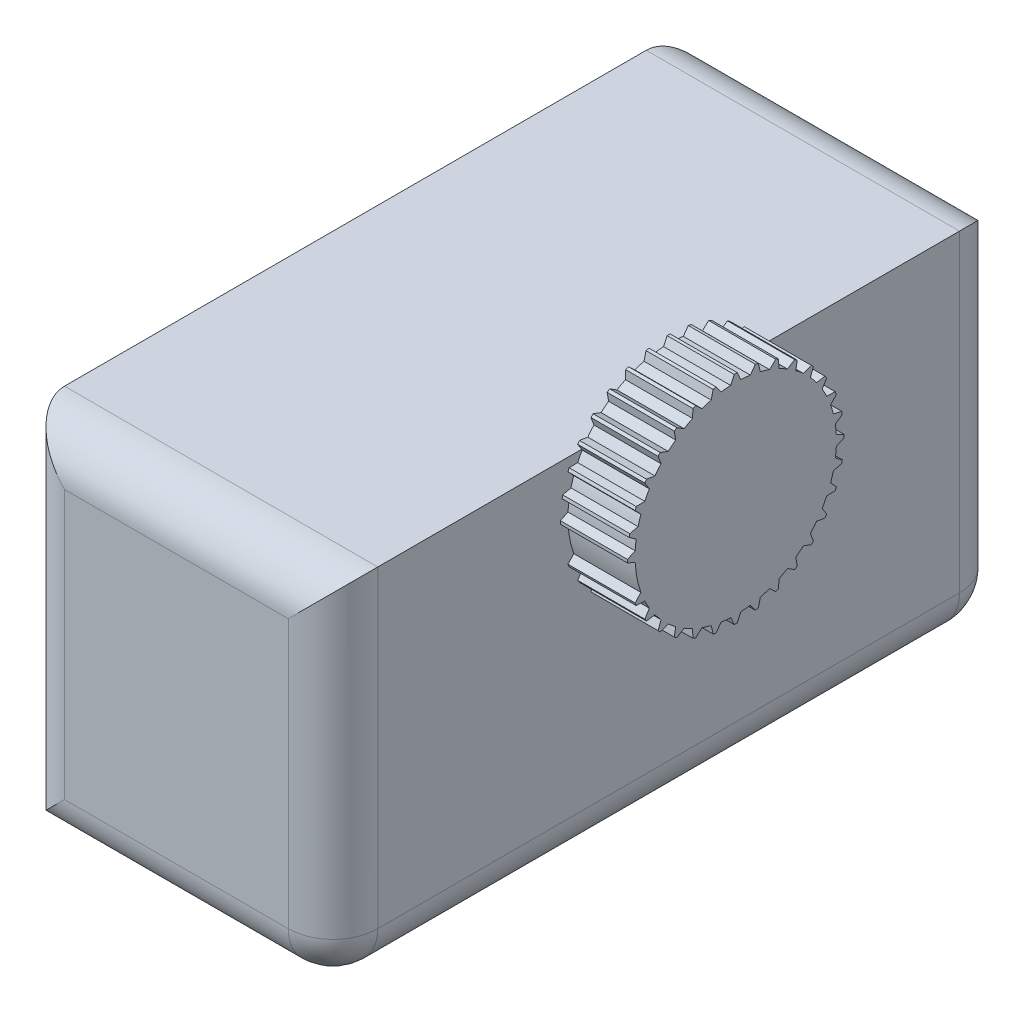
from build123d import *

# Parameters (mm, degrees)
SKETCH1_W                   = 28
SKETCH1_H                   = 32
BOSS_EXTRUDE1_DEPTH         = 30
BOSS_EXTRUDE3_DEPTH         = 6
FILLET1_R                   = 4
TAP_DRILL_FOR_M8_TAP1_D     = 6.8
TAP_DRILL_FOR_M8_TAP1_DEPTH = 5
TAP_DRILL_FOR_M8_TAP1_TIP   = 2.042926105


with BuildPart() as part:
    # Sketch1 → Boss-Extrude1 (new, symmetric)
    with BuildSketch(Plane.XY):
        Rectangle(SKETCH1_W, SKETCH1_H)
    extrude(amount=BOSS_EXTRUDE1_DEPTH, both=True)

    # Sketch2 → Boss-Extrude3 (add)
    with BuildSketch(Plane(origin=(14, 0, 0), x_dir=(0, 0, -1), z_dir=(1, 0, 0))):
        with BuildLine():
            Line((-0.137115518, 20.975970302), (0.137115518, 20.975970302))
            Line((0.137115518, 20.975970302), (0.450893035, 20.282586335))
            ThreePointArc((0.450893035, 20.282586335), (0.882154263, 20.250550667), (1.311378777, 20.197835887))
            Line((1.311378777, 20.197835887), (1.754399647, 20.816681719))
            Line((1.754399647, 20.816681719), (2.023361412, 20.763181898))
            Line((2.023361412, 20.763181898), (2.195837279, 20.021906152))
            ThreePointArc((2.195837279, 20.021906152), (2.612562095, 19.906351149), (3.023255037, 19.77091172))
            Line((3.023255037, 19.77091172), (3.578494218, 20.291437518))
            Line((3.578494218, 20.291437518), (3.83185066, 20.186493844))
            Line((3.83185066, 20.186493844), (3.856396729, 19.425813131))
            ThreePointArc((3.856396729, 19.425813131), (4.242570631, 19.231179507), (4.618949301, 19.01822029))
            Line((4.618949301, 19.01822029), (5.265069263, 19.42042254))
            Line((5.265069263, 19.42042254), (5.493084037, 19.268067939))
            Line((5.493084037, 19.268067939), (5.368757014, 18.517214793))
            ThreePointArc((5.368757014, 18.517214793), (5.709539557, 18.250982208), (6.037139934, 17.968687106))
            Line((6.037139934, 17.968687106), (6.749310649, 18.237109402))
            Line((6.749310649, 18.237109402), (6.943221275, 18.043198777))
            Line((6.943221275, 18.043198777), (6.674798979, 17.331028062))
            ThreePointArc((6.674798979, 17.331028062), (6.95709408, 17.003427685), (7.223326666, 16.662645142))
            Line((7.223326666, 16.662645142), (7.974179812, 16.786972164))
            Line((7.974179812, 16.786972164), (8.126534413, 16.558957391))
            Line((8.126534413, 16.558957391), (7.724332162, 15.912837429))
            ThreePointArc((7.724332162, 15.912837429), (7.937291379, 15.536458759), (8.131925004, 15.150284856))
            Line((8.131925004, 15.150284856), (8.892605716, 15.125738788))
            Line((8.892605716, 15.125738788), (8.997549391, 14.872382346))
            Line((8.997549391, 14.872382346), (8.477023592, 14.317143164))
            ThreePointArc((8.477023592, 14.317143164), (8.612463022, 13.906450223), (8.728018025, 13.489725407))
            Line((8.728018025, 13.489725407), (9.46929377, 13.317249539))
            Line((9.46929377, 13.317249539), (9.522793592, 13.048287775))
            Line((9.522793592, 13.048287775), (8.90394776, 12.605266904))
            ThreePointArc((8.90394776, 12.605266904), (8.95666254, 12.17604239), (8.988698208, 11.744781162))
            Line((8.988698208, 11.744781162), (9.682082175, 11.431003646))
            Line((9.682082175, 11.431003646), (9.682082175, 11.156772609))
            Line((9.682082175, 11.156772609), (8.988698208, 10.842995093))
            ThreePointArc((8.988698208, 10.842995093), (8.95666254, 10.411733864), (8.90394776, 9.982509351))
            Line((8.90394776, 9.982509351), (9.522793592, 9.53948848))
            Line((9.522793592, 9.53948848), (9.46929377, 9.270526716))
            Line((9.46929377, 9.270526716), (8.728018025, 9.098050848))
            ThreePointArc((8.728018025, 9.098050848), (8.612463022, 8.681326032), (8.477023592, 8.270633091))
            Line((8.477023592, 8.270633091), (8.997549391, 7.715393909))
            Line((8.997549391, 7.715393909), (8.892605716, 7.462037467))
            Line((8.892605716, 7.462037467), (8.131925004, 7.437491399))
            ThreePointArc((8.131925004, 7.437491399), (7.937291379, 7.051317496), (7.724332162, 6.674938826))
            Line((7.724332162, 6.674938826), (8.126534413, 6.028818864))
            Line((8.126534413, 6.028818864), (7.974179812, 5.80080409))
            Line((7.974179812, 5.80080409), (7.223326666, 5.925131113))
            ThreePointArc((7.223326666, 5.925131113), (6.95709408, 5.58434857), (6.674798979, 5.256748193))
            Line((6.674798979, 5.256748193), (6.943221275, 4.544577478))
            Line((6.943221275, 4.544577478), (6.749310649, 4.350666852))
            Line((6.749310649, 4.350666852), (6.037139934, 4.619089148))
            ThreePointArc((6.037139934, 4.619089148), (5.709539557, 4.336794047), (5.368757014, 4.070561462))
            Line((5.368757014, 4.070561462), (5.493084037, 3.319708316))
            Line((5.493084037, 3.319708316), (5.265069263, 3.167353714))
            Line((5.265069263, 3.167353714), (4.618949301, 3.569555965))
            ThreePointArc((4.618949301, 3.569555965), (4.242570631, 3.356596748), (3.856396729, 3.161963123))
            Line((3.856396729, 3.161963123), (3.83185066, 2.401282411))
            Line((3.83185066, 2.401282411), (3.578494218, 2.296338737))
            Line((3.578494218, 2.296338737), (3.023255037, 2.816864535))
            ThreePointArc((3.023255037, 2.816864535), (2.612562095, 2.681425106), (2.195837279, 2.565870102))
            Line((2.195837279, 2.565870102), (2.023361412, 1.824594357))
            Line((2.023361412, 1.824594357), (1.754399647, 1.771094536))
            Line((1.754399647, 1.771094536), (1.311378777, 2.389940368))
            ThreePointArc((1.311378777, 2.389940368), (0.882154263, 2.337225587), (0.450893035, 2.30518992))
            Line((0.450893035, 2.30518992), (0.137115518, 1.611805952))
            Line((0.137115518, 1.611805952), (-0.137115518, 1.611805952))
            Line((-0.137115518, 1.611805952), (-0.450893035, 2.30518992))
            ThreePointArc((-0.450893035, 2.30518992), (-0.882154263, 2.337225587), (-1.311378777, 2.389940368))
            Line((-1.311378777, 2.389940368), (-1.754399647, 1.771094536))
            Line((-1.754399647, 1.771094536), (-2.023361412, 1.824594357))
            Line((-2.023361412, 1.824594357), (-2.195837279, 2.565870102))
            ThreePointArc((-2.195837279, 2.565870102), (-2.612562095, 2.681425106), (-3.023255037, 2.816864535))
            Line((-3.023255037, 2.816864535), (-3.578494218, 2.296338737))
            Line((-3.578494218, 2.296338737), (-3.83185066, 2.401282411))
            Line((-3.83185066, 2.401282411), (-3.856396729, 3.161963123))
            ThreePointArc((-3.856396729, 3.161963123), (-4.242570631, 3.356596748), (-4.618949301, 3.569555965))
            Line((-4.618949301, 3.569555965), (-5.265069263, 3.167353714))
            Line((-5.265069263, 3.167353714), (-5.493084037, 3.319708316))
            Line((-5.493084037, 3.319708316), (-5.368757014, 4.070561462))
            ThreePointArc((-5.368757014, 4.070561462), (-5.709539557, 4.336794047), (-6.037139934, 4.619089148))
            Line((-6.037139934, 4.619089148), (-6.749310649, 4.350666852))
            Line((-6.749310649, 4.350666852), (-6.943221275, 4.544577478))
            Line((-6.943221275, 4.544577478), (-6.674798979, 5.256748193))
            ThreePointArc((-6.674798979, 5.256748193), (-6.95709408, 5.58434857), (-7.223326666, 5.925131113))
            Line((-7.223326666, 5.925131113), (-7.974179812, 5.80080409))
            Line((-7.974179812, 5.80080409), (-8.126534413, 6.028818864))
            Line((-8.126534413, 6.028818864), (-7.724332162, 6.674938826))
            ThreePointArc((-7.724332162, 6.674938826), (-7.937291379, 7.051317496), (-8.131925004, 7.437491399))
            Line((-8.131925004, 7.437491399), (-8.892605716, 7.462037467))
            Line((-8.892605716, 7.462037467), (-8.997549391, 7.715393909))
            Line((-8.997549391, 7.715393909), (-8.477023592, 8.270633091))
            ThreePointArc((-8.477023592, 8.270633091), (-8.827067524, 9.538075229), (-8.988698208, 10.842995093))
            Line((-8.988698208, 10.842995093), (-9.682082175, 11.156772609))
            Line((-9.682082175, 11.156772609), (-9.682082175, 11.431003646))
            Line((-9.682082175, 11.431003646), (-8.988698208, 11.744781162))
            ThreePointArc((-8.988698208, 11.744781162), (-8.95666254, 12.17604239), (-8.90394776, 12.605266904))
            Line((-8.90394776, 12.605266904), (-9.522793592, 13.048287775))
            Line((-9.522793592, 13.048287775), (-9.46929377, 13.317249539))
            Line((-9.46929377, 13.317249539), (-8.728018025, 13.489725407))
            ThreePointArc((-8.728018025, 13.489725407), (-8.612463022, 13.906450223), (-8.477023592, 14.317143164))
            Line((-8.477023592, 14.317143164), (-8.997549391, 14.872382346))
            Line((-8.997549391, 14.872382346), (-8.892605716, 15.125738788))
            Line((-8.892605716, 15.125738788), (-8.131925004, 15.150284856))
            ThreePointArc((-8.131925004, 15.150284856), (-7.937291379, 15.536458759), (-7.724332162, 15.912837429))
            Line((-7.724332162, 15.912837429), (-8.126534413, 16.558957391))
            Line((-8.126534413, 16.558957391), (-7.974179812, 16.786972164))
            Line((-7.974179812, 16.786972164), (-7.223326666, 16.662645142))
            ThreePointArc((-7.223326666, 16.662645142), (-6.95709408, 17.003427685), (-6.674798979, 17.331028062))
            Line((-6.674798979, 17.331028062), (-6.943221275, 18.043198777))
            Line((-6.943221275, 18.043198777), (-6.749310649, 18.237109402))
            Line((-6.749310649, 18.237109402), (-6.037139934, 17.968687106))
            ThreePointArc((-6.037139934, 17.968687106), (-5.709539557, 18.250982208), (-5.368757014, 18.517214793))
            Line((-5.368757014, 18.517214793), (-5.493084037, 19.268067939))
            Line((-5.493084037, 19.268067939), (-5.265069263, 19.42042254))
            Line((-5.265069263, 19.42042254), (-4.618949301, 19.01822029))
            ThreePointArc((-4.618949301, 19.01822029), (-4.242570631, 19.231179507), (-3.856396729, 19.425813131))
            Line((-3.856396729, 19.425813131), (-3.83185066, 20.186493844))
            Line((-3.83185066, 20.186493844), (-3.578494218, 20.291437518))
            Line((-3.578494218, 20.291437518), (-3.023255037, 19.77091172))
            ThreePointArc((-3.023255037, 19.77091172), (-2.612562095, 19.906351149), (-2.195837279, 20.021906152))
            Line((-2.195837279, 20.021906152), (-2.023361412, 20.763181898))
            Line((-2.023361412, 20.763181898), (-1.754399647, 20.816681719))
            Line((-1.754399647, 20.816681719), (-1.311378777, 20.197835887))
            ThreePointArc((-1.311378777, 20.197835887), (-0.882154263, 20.250550667), (-0.450893035, 20.282586335))
            Line((-0.450893035, 20.282586335), (-0.137115518, 20.975970302))
        make_face()
    extrude(amount=BOSS_EXTRUDE3_DEPTH)

    # Fillet1
    fillet1_edges = [part.edges().sort_by_distance(p)[0] for p in [
        (14, 0, 30),
        (0, 16, 30),
        (-14, 0, 30),
        (0, 16, -30),
        (14, 0, -30),
        (0, -16, -30),
        (-14, 0, -30),
        (14, -16, 0),
        (0, -16, 30),
    ]]
    fillet(fillet1_edges, radius=FILLET1_R)

    # Tap Drill for M8 Tap1
    with Locations(Plane.XZ.offset(16)):
        with Locations((-2, 10), (-2, -10)):
            Hole(TAP_DRILL_FOR_M8_TAP1_D / 2, depth=TAP_DRILL_FOR_M8_TAP1_DEPTH)
            with Locations((0, 0, -(TAP_DRILL_FOR_M8_TAP1_DEPTH + TAP_DRILL_FOR_M8_TAP1_TIP / 2))):  # 118° drill point
                Cone(0, TAP_DRILL_FOR_M8_TAP1_D / 2, TAP_DRILL_FOR_M8_TAP1_TIP, mode=Mode.SUBTRACT)


solid = part.part
